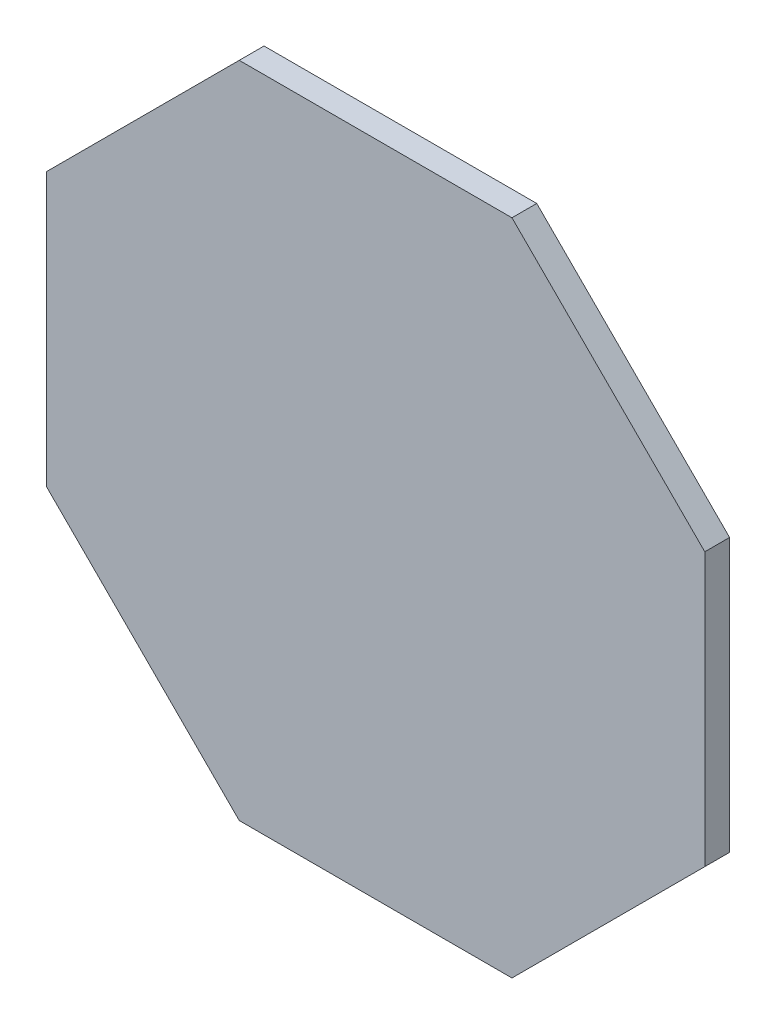
SolidWorks part; units mm, degrees
ref_plane "Front Plane" through (0, 0, 0) normal (0, 0, 1) x (1, 0, 0)
ref_plane "Top Plane" through (0, 0, 0) normal (0, 1, 0) x (1, 0, 0)
ref_plane "Right Plane" through (0, 0, 0) normal (1, 0, 0) x (0, 0, -1)
other "Configuration Table"
sketch "Sketch1" plane through (0, 0, 0) normal (0, 0, 1) x (1, 0, 0)
  circle A0 centre (-659.8842, -20) radius 20
  circle A1 centre (-539.8842, -20) radius 20
  circle A2 centre (-539.8842, -160) radius 20
  circle A3 centre (-659.8842, -20) radius 25
  circle A4 centre (-539.8842, -20) radius 25
  circle A5 centre (-539.8842, -160) radius 25
  dimension "D1" = 5
extrude "Boss-Extrude1" add sketch "Sketch1" against normal blind 10
sketch "Sketch2" plane through (0, 0, 0) normal (0, 0, 1) x (1, 0, 0)
  line L0 (-659.8842, -20) -> (-539.8842, -160) construction
  line L1 (-599.8842, -90) -> (-539.8842, -20) construction
  line L3 (-544.8842, -222.7817) -> (-467.1025, -145)
  line L4 (-467.1025, -145) -> (-467.1025, -35)
  line L5 (-467.1025, -35) -> (-544.8842, 42.7817)
  line L6 (-544.8842, 42.7817) -> (-654.8842, 42.7817)
  line L7 (-654.8842, 42.7817) -> (-732.6659, -35)
  line L8 (-732.6659, -35) -> (-732.6659, -145)
  line L9 (-732.6659, -145) -> (-654.8842, -222.7817)
  line L10 (-654.8842, -222.7817) -> (-544.8842, -222.7817)
  circle A0 centre (-599.8842, -90) radius 132.7817 construction
  dimension "D1" = 110
extrude "Boss-Extrude2" add sketch "Sketch2" along normal blind 10
